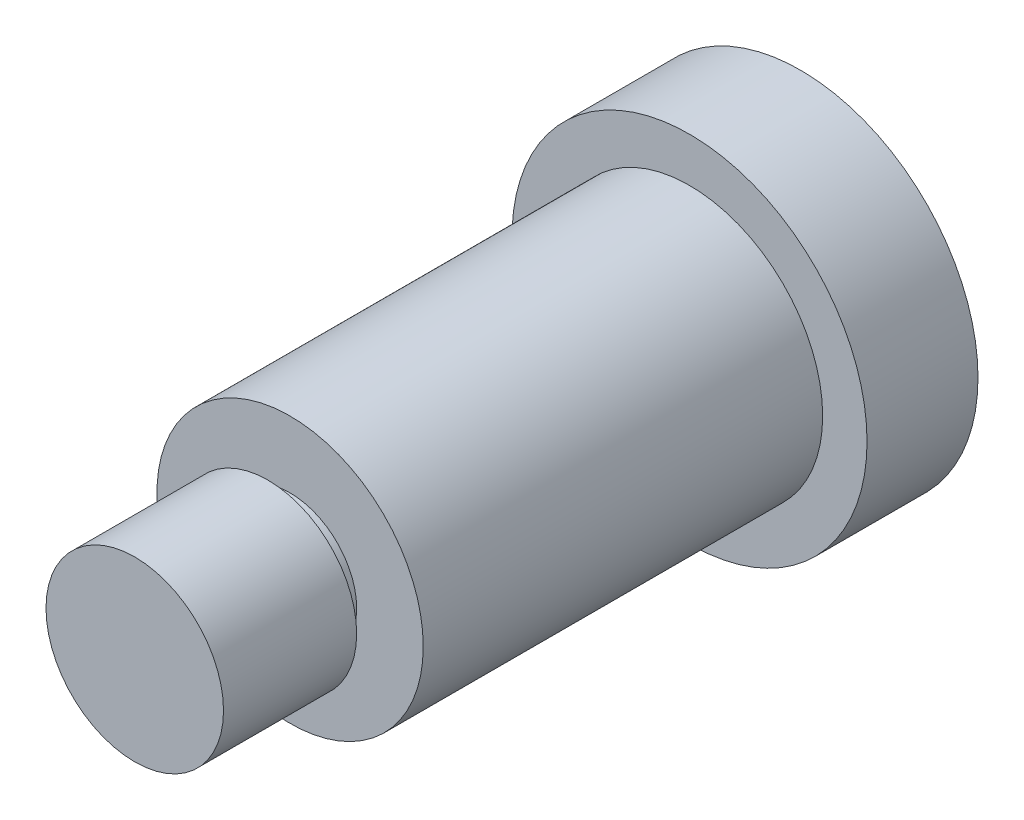
from build123d import *


with BuildPart() as part:
    # Sketch1 → Revolve1 (revolve)
    with BuildSketch(Plane(origin=(0, 0, 0), x_dir=(0, 0, -1), z_dir=(1, 0, 0)), mode=Mode.PRIVATE) as revolve1_sk:
        Polygon((30, 0), (30, 8), (25, 8), (25, 6), (7, 6), (7, 3), (6, 3), (6, 4), (0, 4), (0, 0), align=None)
    revolve(revolve1_sk.sketch.rotate(Axis((0, 0, 0), (0, 0, -1)), 90), axis=Axis((0, 0, 0), (0, 0, -1)))


solid = part.part
